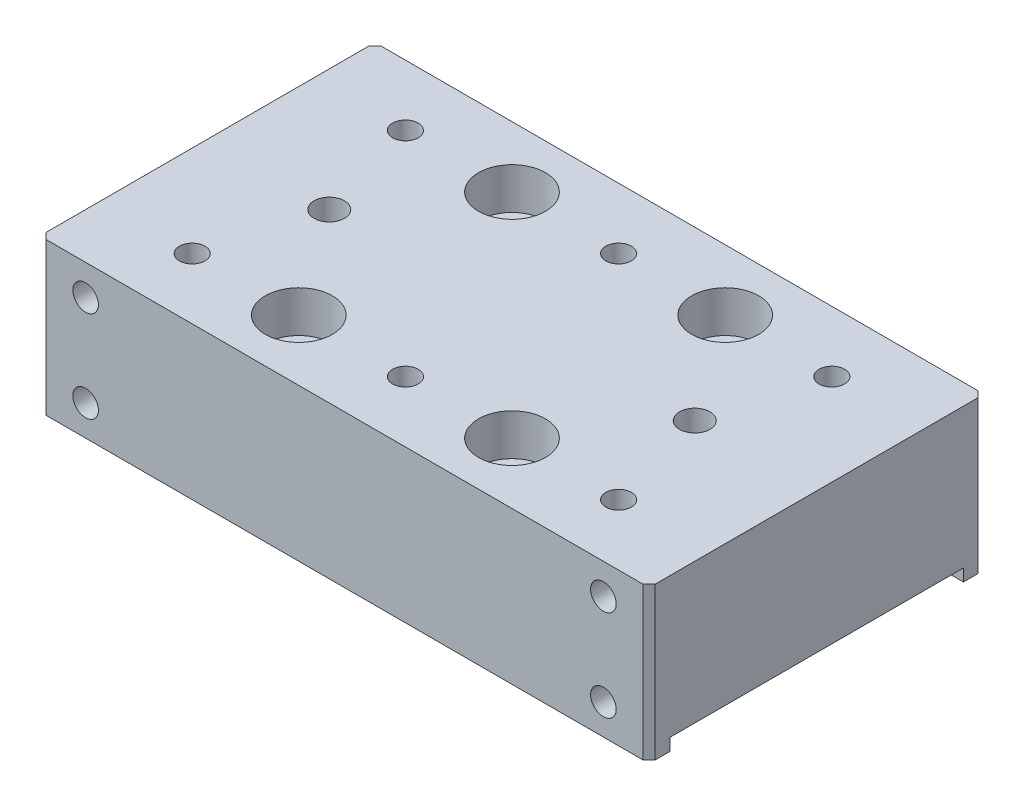
from build123d import *

# Parameters (mm, degrees)
SKETCH_1_W                = 100
SKETCH_1_H                = 55
EXTRUDE_1_DEPTH           = 25
SKETCH_2_W                = 48.2
SKETCH_2_H                = 4
CUT_EXTRUDE_1_DEPTH       = 107.682941467
HOLE_WIZARD_M5_1_D        = 4.2
HOLE_WIZARD_M5_1_DEPTH    = 12.4
HOLE_WIZARD_M5_1_TIP      = 1.2618073
CHAMFER_1_SIZE            = 1
HOLE_WIZARD_0_D           = 6.6
HOLE_WIZARD_0_DEPTH       = 40
HOLE_WIZARD_0_CBORE_D     = 11
HOLE_WIZARD_0_CBORE_DEPTH = 6.8
HOLE_WIZARD_0_TIP         = 1.982840043
HOLE_WIZARD_M5_2_D        = 4.2
HOLE_WIZARD_M5_2_DEPTH    = 12.4
HOLE_WIZARD_M5_2_TIP      = 1.2618073
MM_1_D                    = 5
MM_1_DEPTH                = 12.4
MM_1_TIP                  = 1.502151548


with BuildPart() as part:
    # 草图1 → 凸台-拉伸1 (new body)
    with BuildSketch(Plane(origin=(0, 0, 0), x_dir=(1, 0, 0), z_dir=(0, 1, 0))):
        Rectangle(SKETCH_1_W, SKETCH_1_H)
    extrude(amount=EXTRUDE_1_DEPTH)

    # 草图2 → 切除-拉伸1 (cut, through all)
    with BuildSketch(Plane(origin=(50, 0, 0), x_dir=(0, 0, -1), z_dir=(1, 0, 0))):
        Rectangle(SKETCH_2_W, SKETCH_2_H)
    extrude(amount=-CUT_EXTRUDE_1_DEPTH, mode=Mode.SUBTRACT)

    # M5 螺纹孔1
    with Locations(Plane.XY.offset(27.5)):
        with Locations((42.5, 20), (42.5, 5), (-42.5, 20), (-42.5, 5)):
            Hole(HOLE_WIZARD_M5_1_D / 2, depth=HOLE_WIZARD_M5_1_DEPTH)
            with Locations((0, 0, -(HOLE_WIZARD_M5_1_DEPTH + HOLE_WIZARD_M5_1_TIP / 2))):  # 118° drill point
                Cone(0, HOLE_WIZARD_M5_1_D / 2, HOLE_WIZARD_M5_1_TIP, mode=Mode.SUBTRACT)

    # 倒角1
    chamfer_1_edges = [part.edges().sort_by_distance(p)[0] for p in [
        (50, 12.5, 27.5),
        (-50, 12.5, 27.5),
        (-50, 12.5, -27.5),
        (50, 12.5, -27.5),
    ]]
    chamfer(chamfer_1_edges, length=CHAMFER_1_SIZE)

    # 打孔尺寸(%根据)内六角圆柱头螺钉的类型0
    with Locations(Plane(origin=(0, 25, 0), x_dir=(1, 0, 0), z_dir=(0, 1, 0))):
        with Locations((-17.499999996, 17.499999996), (17.500000004, 17.499999996), (-17.499999996, -17.500000004), (17.500000004, -17.500000004)):
            CounterBoreHole(HOLE_WIZARD_0_D / 2, HOLE_WIZARD_0_CBORE_D / 2, HOLE_WIZARD_0_CBORE_DEPTH, depth=HOLE_WIZARD_0_DEPTH)
            with Locations((0, 0, -(HOLE_WIZARD_0_DEPTH + HOLE_WIZARD_0_TIP / 2))):  # 118° drill point
                Cone(0, HOLE_WIZARD_0_D / 2, HOLE_WIZARD_0_TIP, mode=Mode.SUBTRACT)

    # M5 螺纹孔2
    with Locations(Plane(origin=(0, 25, 0), x_dir=(1, 0, 0), z_dir=(0, 1, 0))):
        with Locations((-35, 17.5), (-35, -17.5), (35, 17.5), (35, -17.5), (0, 17.5), (0, -17.5)):
            Hole(HOLE_WIZARD_M5_2_D / 2, depth=HOLE_WIZARD_M5_2_DEPTH)
            with Locations((0, 0, -(HOLE_WIZARD_M5_2_DEPTH + HOLE_WIZARD_M5_2_TIP / 2))):  # 118° drill point
                Cone(0, HOLE_WIZARD_M5_2_D / 2, HOLE_WIZARD_M5_2_TIP, mode=Mode.SUBTRACT)

    # 大小mm 暗销孔1
    with Locations(Plane(origin=(0, 25, 0), x_dir=(1, 0, 0), z_dir=(0, 1, 0))):
        with Locations((-30, 0), (30, 0)):
            Hole(MM_1_D / 2, depth=MM_1_DEPTH)
            with Locations((0, 0, -(MM_1_DEPTH + MM_1_TIP / 2))):  # 118° drill point
                Cone(0, MM_1_D / 2, MM_1_TIP, mode=Mode.SUBTRACT)


solid = part.part
